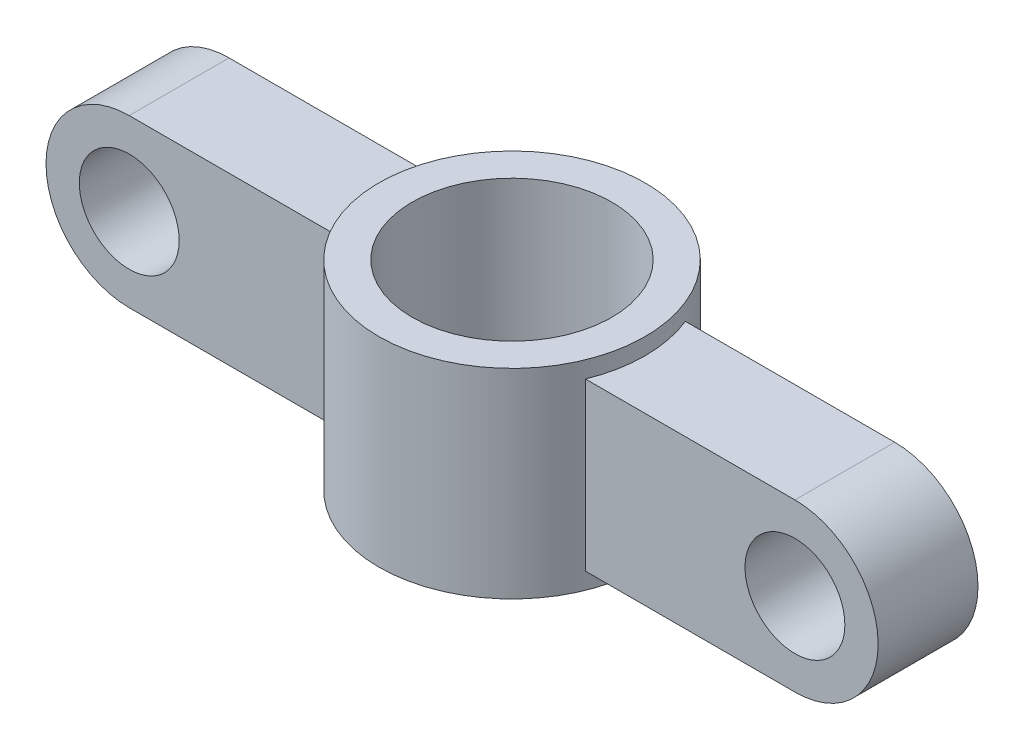
SolidWorks part; units mm, degrees
ref_plane "Front Plane" through (0, 0, 0) normal (0, 0, 1) x (1, 0, 0)
ref_plane "Top Plane" through (0, 0, 0) normal (0, 1, 0) x (1, 0, 0)
ref_plane "Right Plane" through (0, 0, 0) normal (1, 0, 0) x (0, 0, -1)
other "Configuration Table"
sketch "Sketch1" plane through (0, 0, 0) normal (0, 1, 0) x (1, 0, 0)
  circle A0 centre (0, 0) radius 3
  circle A1 centre (0, 0) radius 4
  dimension "D1" = 6
  dimension "D2" = 8
extrude "Boss-Extrude1" add sketch "Sketch1" along normal blind 6
sketch "Sketch2" plane through (0, 0, 0) normal (0, 0, 1) x (1, 0, 0)
  line L0 (-10, 5.5) -> (-3, 5.5)
  line L2 (-3, 5.5) -> (-3, 0.5)
  line L3 (-3, 0.5) -> (-10, 0.5)
  line L4 (-4, 6) -> (-4, 0) construction
  line L5 (0, 0) -> (0, 6) construction
  line L6 (4, 6) -> (-4, 6) construction
  line L7 (-4, 0) -> (4, 0) construction
  line L8 (3, 0.5) -> (10, 0.5)
  line L9 (3, 5.5) -> (3, 0.5)
  line L10 (10, 5.5) -> (3, 5.5)
  circle A0 centre (-10, 3) radius 1.5
  circle A1 centre (-10, 3) radius 2.5
  circle A2 centre (10, 3) radius 2.5
  circle A3 centre (10, 3) radius 1.5
  dimension "D3" = 7
  dimension "D4" = 3
  dimension "D5" = 5
  dimension "D1" = 1
  dimension "D2" = 3
extrude "Boss-Extrude2" add sketch "Sketch2" along normal mid plane 3 contours A1 L3 L2 L0 | A1 A0 | L8 A2 L10 L9 | A2 A3
